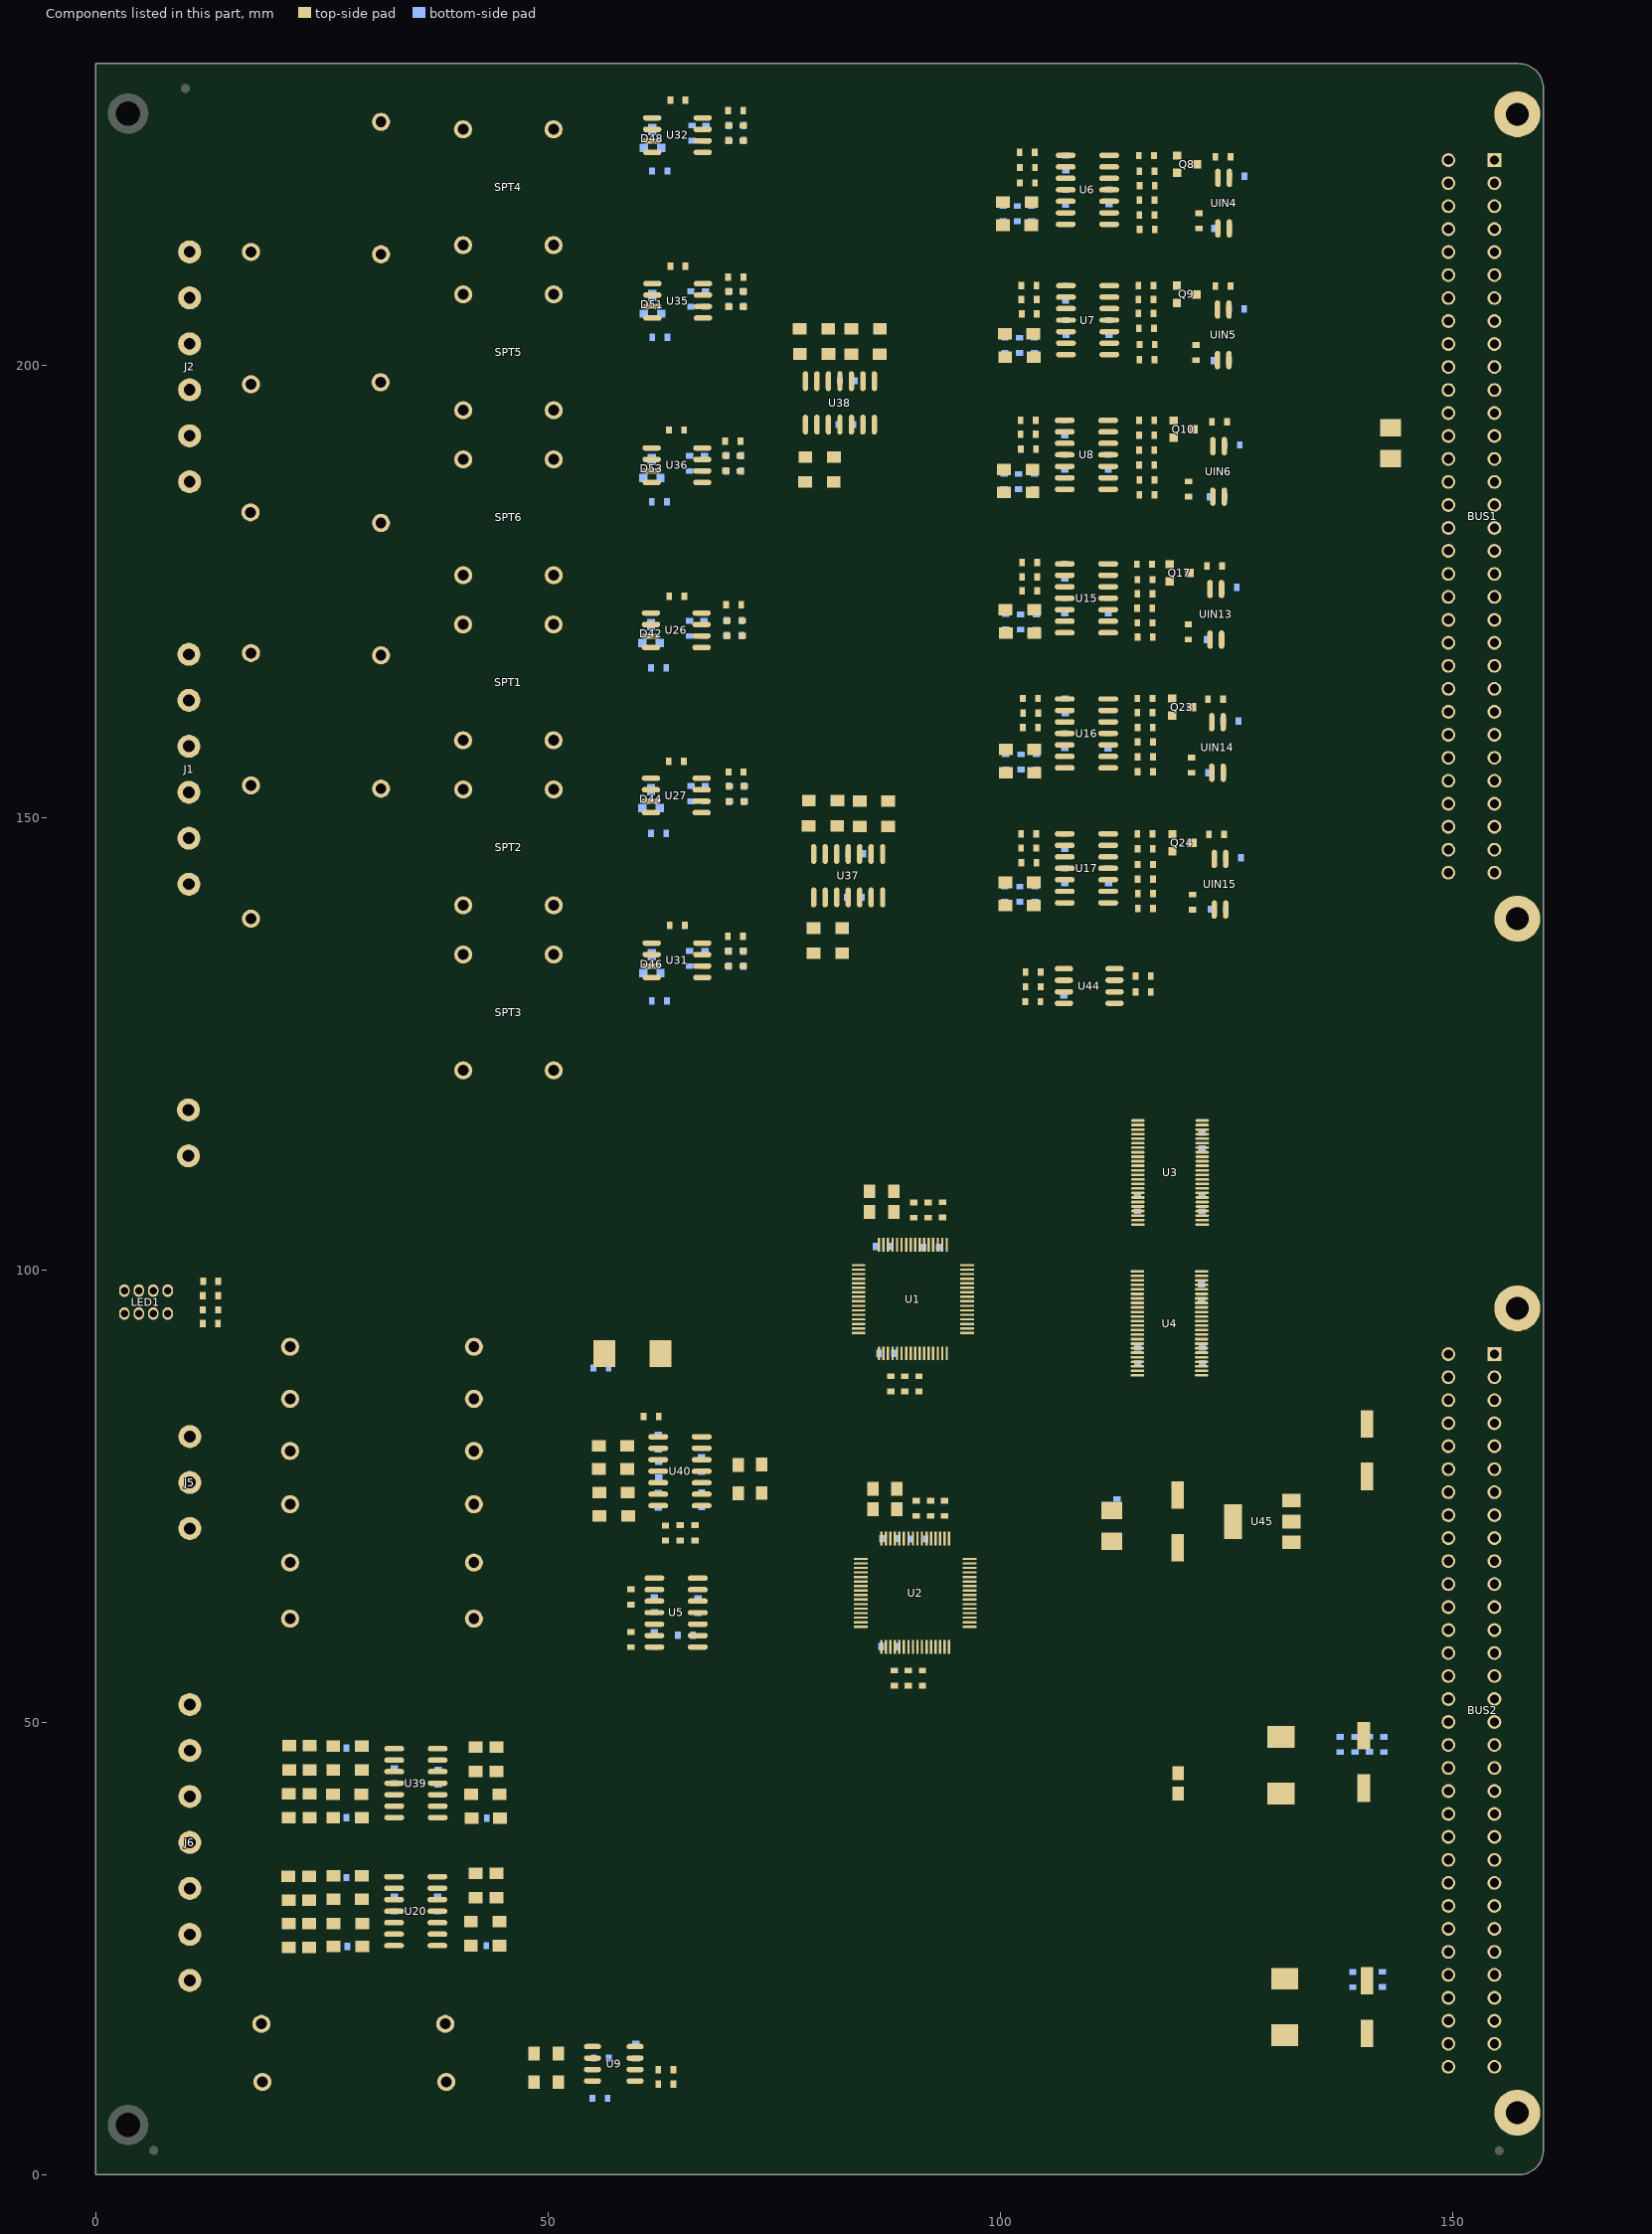
[diagram p0: the components of this part, seen from the top]
# Altium PCB MISC80584.PCBDoc (part 7 of 7)
Units mm, origin at the board's own origin, x right, y up, seen from the top; angles counter-clockwise.
Board outline 160.02 x 233.3 mm, 4 copper layers (TopLayer, GND, POWER, BottomLayer); 386 components, 266 nets, 1374 pads, 640 vias.

## Polygon pours and split planes (outlines as drawn) (continued)
AGND on TopLayer "Top Layer-No Net" (solid, remove dead copper): -1.784,125.495 -1.784,13.481 0.705,10.992 1.061,10.636 3.575,10.636 7.69,10.636 8.35,9.976 8.681,9.646 8.681,8.528 8.681,3.016 9.163,2.534 9.57,2.127 10.713,2.127 151.784,2.127 152.749,3.093 152.902,3.245 152.902,6.141 152.902,10.103 153.715,10.916 153.74,10.941 157.067,10.941 157.499,10.941 157.982,11.424 158.261,11.703 158.261,14.142 158.261,223.361 157.575,224.047 157.321,224.301 156.305,224.301 154.553,224.301 153.842,225.012 153.003,225.851 153.003,227.121 153.003,230.626 152.089,231.54 151.86,231.769 149.955,231.769 59.582,231.769 59.277,231.464 58.134,230.321 58.134,226.105 58.134,118.231 57.245,117.342 56.509,116.605 51.581,116.605 23.717,116.605 22.574,117.748 22.447,117.875 22.447,120.491 22.447,126.079 20.72,127.807 20.238,128.289 17.698,128.289 1.213,128.289 -0.514,126.562 -1.581,125.495 -1.784,125.495
GND on TopLayer "Top Layer-No Net" (solid, remove dead copper): 107.848,75.413 107.848,45.06 108.534,44.374 109.322,43.586 120.929,43.586 121.183,43.84 121.336,43.993 121.336,45.212 121.336,58.979 123.901,61.544 124.003,61.646 129.057,61.646 135.89,61.646 137.033,62.789 137.871,63.627 137.871,65.964 137.871,69.113 137.871,69.774 137.109,70.536 136.957,70.688 132.817,70.688 130.734,70.688 129.769,69.723 128.499,68.453 124.968,68.453 123.8,68.453 121.742,70.51 121.158,71.095 113.767,71.095 110.642,71.095 110.439,71.298 109.957,71.78 109.957,72.517 109.957,78.207 110.871,79.121 111.379,79.629 111.608,79.858 130.505,79.858 130.988,80.34 131.801,81.153 139.624,81.153 142.088,81.153 142.773,81.839 143.154,82.22 149.25,82.22 155.499,82.22 155.778,82.499 155.931,82.652 155.931,83.541 155.931,91.567 155.702,91.796 155.651,91.846 154.559,91.846 130.531,91.846 127.076,88.392 125.679,86.995 120.345,86.995 112.878,86.995 110.134,84.252 107.848,81.966 107.848,75.413
+15V on TopLayer "Top Layer-No Net" (solid, remove dead copper): 51.867,91.897 51.867,89.484 51.867,88.976 52.273,88.57 52.756,88.087 54.127,88.087 57.353,88.087 57.582,88.316 57.81,88.544 57.81,89.332 57.81,92.837 57.252,93.396 57.175,93.472 55.982,93.472 52.705,93.472 52.146,92.913 51.867,92.634 51.867,91.897
+5V on TopLayer "TopLayer-No Net" (solid, remove dead copper, pour order 1002): 141.072,189.56 141.072,186.665 144.018,183.718 144.094,183.642 154.432,183.642 155.346,183.642 155.6,183.896 155.956,184.252 155.956,185.293 155.956,194.869 155.55,195.275 155.346,195.478 155.296,195.529 148.615,195.529 147.447,195.529 147.168,195.25 146.888,194.97 146.888,194.513 146.888,191.338 146.685,191.135 146.304,190.754 144.856,190.754 141.453,190.754 141.224,190.525 141.072,190.373 141.072,189.56
+5V on TopLayer "TopLayer-No Net" (solid, remove dead copper, pour order 1001): 130.962,76.505 130.962,73.99 130.962,73.889 131.14,73.711 131.801,73.711 133.426,73.711 138.074,73.711 138.227,73.558 139.751,72.034 153.873,72.034 155.321,72.034 155.55,72.263 155.905,72.619 155.905,73.177 155.905,80.772 155.55,81.128 155.296,81.382 155.245,81.432 155.219,81.407 146.406,81.407 145.415,81.407 143.967,79.959 142.977,78.969 140.538,78.969 132.283,78.969 132.207,78.969 132.08,78.969 131.343,78.232 131.039,77.927 130.962,77.851 130.962,76.505
+3.3V on TopLayer "TopLayer-No Net" (solid, remove dead copper, pour order 1000): 110.642,76.429 110.642,74.143 110.642,73.482 110.642,72.923 110.642,72.72 111.049,72.314 114.046,72.314 115.138,73.406 119.888,73.406 122.301,73.406 122.987,72.72 123.419,72.288 123.419,71.73 123.419,70.587 123.825,70.18 124.308,69.698 124.689,69.698 128.295,69.698 129.337,70.739 129.972,71.374 131.877,71.374 133.172,71.374 133.299,71.501 133.375,71.577 133.375,71.704 133.375,72.923 133.274,73.025 133.223,73.076 133.172,73.127 129.997,73.127 124.257,78.867 112.192,78.867 111.506,78.867 110.769,78.13 110.668,78.029 110.642,78.003 110.642,76.454
+5VREF on TopLayer "Top Layer-No Net" (solid, remove dead copper, pour order 1000): 116.256,132.867 116.256,132.131 116.256,132.029 116.485,131.902 116.669,131.801 117.495,131.801 120.202,131.801 120.431,131.928 120.523,131.978 120.523,132.563 120.523,132.969 120.248,133.121 120.202,133.147 119.238,133.147 116.531,133.147 116.348,133.045 116.256,132.994 116.256,132.867
+15V on TopLayer "TopLayer-No Net" (solid, remove dead copper, pour order 1000): 128.397,50.47 128.397,48.26 128.397,47.549 128.397,47.447 129.032,46.812 129.057,46.787 129.235,46.609 155.372,46.609 155.524,46.609 155.575,46.609 156.337,47.371 156.54,47.574 156.54,49.428 156.54,57.633 155.854,58.318 155.6,58.572 154.788,58.572 147.955,58.572 147.168,57.785 142.926,53.543 142.545,53.162 131.445,53.162 129.997,53.162 129.515,52.68 128.397,51.562 128.397,50.47
-15V on TopLayer "TopLayer-No Net" (solid, remove dead copper, pour order 1001): 128.473,24.282 128.473,21.514 128.473,20.803 128.829,20.447 129.438,19.837 140.208,19.837 145.644,19.837 146.685,18.796 146.863,18.618 146.888,18.593 155.448,18.593 155.55,18.593 155.829,18.872 156.718,19.761 156.718,32.233 156.718,32.512 156.718,32.588 155.931,33.376 155.88,33.426 153.086,33.426 148.336,33.426 146.964,32.055 143.129,28.219 139.37,28.219 130.734,28.219 129.159,26.645 128.473,25.959 128.473,24.282
AGND on BottomLayer "Top Layer-No Net" (solid, remove dead copper): -1.778,125.508 -1.778,13.494 0.711,11.005 1.067,10.649 3.581,10.649 7.696,10.649 8.357,9.989 8.687,9.659 8.687,8.541 8.687,3.029 9.169,2.547 9.576,2.14 10.719,2.14 151.79,2.14 152.756,3.106 152.908,3.258 152.908,6.154 152.908,10.116 153.721,10.929 153.746,10.954 157.074,10.954 157.505,10.954 157.988,11.437 158.267,11.716 158.267,14.155 158.267,223.374 157.582,224.06 157.328,224.314 156.312,224.314 154.559,224.314 153.848,225.025 153.01,225.864 153.01,227.134 153.01,230.639 152.095,231.553 151.867,231.782 149.962,231.782 59.588,231.782 59.284,231.477 58.141,230.334 58.141,226.118 58.141,118.244 57.252,117.355 56.515,116.618 51.587,116.618 23.724,116.618 22.581,117.761 22.454,117.888 22.454,120.504 22.454,126.092 20.726,127.82 20.244,128.302 17.704,128.302 1.219,128.302 -0.508,126.575 -1.575,125.508 -1.778,125.508
+5VREF on BottomLayer "Top Layer-No Net" (solid, remove dead copper, pour order 1001): 118.694,132.994 118.694,132.156 118.77,132.08 119.05,131.801 119.532,131.801 120.548,131.801 120.752,132.004 120.828,132.08 120.828,132.436 120.828,133.426 120.625,133.629 120.498,133.756 120.193,133.756 119.964,133.756 119.761,133.553 119.558,133.35 119.38,133.35 118.897,133.35 118.77,133.223 118.694,133.147 118.694,133.02
+15V on BottomLayer "TopLayer-No Net" (solid, remove dead copper, pour order 1002): 136.754,49.911 136.754,48.336 136.906,48.184 137.058,48.031 137.084,48.057 141.351,48.057 142.824,48.057 142.9,48.133 143.002,48.235 143.002,48.463 143.002,51.206 142.418,51.791 142.265,51.943 140.843,51.943 138.201,51.943 138.024,51.765 136.754,50.495 136.754,49.911
-15V on BottomLayer "TopLayer-No Net" (solid, remove dead copper, pour order 1003): 138.227,24.536 138.227,22.327 138.324,22.2 138.558,21.895 139.025,21.895 142.819,21.895 143.014,22.149 143.053,22.2 143.053,22.555 143.053,24.689 142.644,25.222 138.752,25.222 138.227,24.536
AGND on GND (split plane): 157.495,232.808 157.686,232.782 157.874,232.741 158.058,232.683 158.236,232.609 158.407,232.52 158.569,232.416 158.722,232.299 158.864,232.169 158.995,232.027 159.112,231.874 159.216,231.711 159.305,231.54 159.378,231.362 159.436,231.178 159.478,230.99 159.503,230.799 159.511,230.621 159.51,230.607 159.51,221.643 125.578,221.643 125.511,221.634 125.45,221.608 125.396,221.568 120.469,216.64 120.428,216.587 120.403,216.525 120.394,216.459 120.394,126.116 114.092,119.814 95.072,119.814 95.006,119.805 94.962,119.787 94.944,119.78 94.891,119.739 89.354,114.202 89.313,114.149 89.288,114.087 89.279,114.021 89.279,102.798 88.82,102.34 88.78,102.287 88.754,102.225 88.745,102.159 88.745,101.224 88.26,100.739 87.152,100.739 86.567,101.324 86.513,101.365 86.452,101.39 86.385,101.399 84.785,101.399 84.719,101.39 84.657,101.365 84.604,101.324 84.563,101.271 84.554,101.249 83.791,100.486 83.751,100.433 83.725,100.371 83.716,100.305 83.716,87.046 83.725,86.979 83.751,86.918 83.791,86.865 89.66,80.996 89.66,68.762 89.378,68.481 84.125,68.481 84.058,68.472 83.997,68.446 83.944,68.406 80.388,64.85 80.347,64.796 80.321,64.735 80.313,64.668 80.313,55.829 80.321,55.763 80.347,55.701 80.388,55.648 80.402,55.637 80.413,55.623 90.725,45.31 90.779,45.27 90.84,45.244 90.907,45.235 118.364,45.235 118.43,45.244 118.492,45.27 118.545,45.31 139.273,66.038 159.51,66.038 159.51,2.743 159.511,2.729 159.503,2.551 159.478,2.36 159.436,2.171 159.378,1.988 159.305,1.809 159.216,1.639 159.112,1.476 158.995,1.323 158.864,1.181 158.722,1.051 158.569,0.933 158.407,0.83 158.236,0.741 158.058,0.667 157.874,0.609 157.686,0.567 157.495,0.542 157.316,0.534 157.302,0.536 0.51,0.536 0.51,129.669 0.864,130.023 23.825,130.023 24.46,129.388 24.46,119.659 25.603,118.516 44.577,118.516 44.679,118.618 44.679,232.029 45.464,232.814 157.302,232.814 157.316,232.815
GND on GND (split plane): 159.51,66.55 139.167,66.55 139.1,66.541 139.039,66.516 138.985,66.475 118.258,45.748 91.013,45.748 80.825,55.935 80.825,64.562 84.231,67.968 89.484,67.968 89.551,67.977 89.612,68.003 89.665,68.043 90.097,68.475 90.138,68.528 90.163,68.59 90.172,68.656 90.172,81.102 90.163,81.169 90.145,81.212 90.138,81.23 90.097,81.283 84.229,87.152 84.229,100.198 84.917,100.887 86.279,100.887 86.865,100.301 86.918,100.261 86.936,100.253 86.979,100.235 87.046,100.226 88.367,100.226 88.433,100.235 88.495,100.261 88.548,100.301 89.183,100.936 89.223,100.989 89.242,101.033 89.249,101.051 89.258,101.117 89.258,102.053 89.716,102.511 89.757,102.564 89.77,102.595 89.782,102.626 89.791,102.692 89.791,113.914 95.178,119.302 114.198,119.302 114.265,119.31 114.326,119.336 114.38,119.377 120.831,125.828 120.872,125.881 120.897,125.943 120.906,126.009 120.906,216.353 125.684,221.13 159.51,221.13
+15V on POWER (split plane): 313 vertices, not listed, extent 27.917,11.483 159.511,232.815
-15V on POWER (split plane): 188 vertices, not listed, extent 0.51,0.534 159.511,232.814
+5V on POWER (split plane): 189 vertices, not listed, extent 77.955,39.499 159.51,215.898
+3.3V on POWER (split plane): 120.673,105.105 120.682,105.039 120.708,104.977 120.748,104.924 124.636,101.037 124.636,99.014 123.719,98.097 121.336,98.097 121.269,98.088 121.226,98.07 121.208,98.063 121.155,98.022 120.113,96.981 120.073,96.927 120.047,96.866 120.038,96.799 120.038,76.581 120.04,76.568 120.038,76.556 120.038,71.15 100.783,51.894 89.26,51.894 87.785,53.37 87.785,56.587 93.425,62.227 93.465,62.28 93.491,62.341 93.5,62.408 93.5,72.746 93.491,72.812 93.473,72.856 93.465,72.874 93.425,72.927 91.315,75.036 91.315,76.657 91.306,76.724 91.281,76.785 91.24,76.838 88.14,79.938 88.14,89.2 89.894,90.954 89.935,91.007 89.942,91.025 89.96,91.069 89.969,91.135 89.969,97.328 93.577,100.936 93.618,100.989 93.625,101.007 93.643,101.051 93.652,101.117 93.652,104.394 93.643,104.46 93.625,104.504 93.618,104.522 93.577,104.575 92.536,105.617 92.482,105.657 92.421,105.683 92.354,105.692 83.263,105.692 83.263,108.301 92.105,117.143 120.673,117.143

## Keep-outs
KeepOutLayer:
  lines w0.127: 4.394,130.073 cw(c4.394,130.835) 4.394,131.597 24.663,131.597 26.086,130.175 26.086,120.345 26.391,120.04 35.687,120.04 43.155,120.04 43.155,126.086 cw(c43.917,126.086) 44.679,126.086 44.679,118.516 35.687,118.516 25.578,118.516 24.46,119.634 24.46,129.362 23.749,130.073 4.42,130.073 ; 37.109,228.016 43.155,228.016 43.155,220.548 ccw(c43.917,220.548) 44.679,220.548 44.679,229.54 37.109,229.54 ; 37.16,228.016 cw(c37.16,228.778) 37.16,229.54 ; 43.155,131.928 ccw(c43.917,131.928) 44.679,131.928 44.679,143.815 ccw(c43.917,143.815) 43.155,143.815 43.155,131.928 ; 43.155,149.835 ccw(c43.917,149.835) 44.679,149.835 44.679,161.722 ccw(c43.917,161.722) 43.155,161.722 43.155,149.835 ; 43.155,165.837 ccw(c43.917,165.837) 44.679,165.837 44.679,180.797 ccw(c43.917,180.797) 43.155,180.797 43.155,173.228 43.155,165.837 ; 43.155,186.639 ccw(c43.917,186.639) 44.679,186.639 44.679,198.526 ccw(c43.917,198.526) 43.155,198.526 43.155,186.639 ; 43.155,204.546 ccw(c43.917,204.546) 44.679,204.546 44.679,216.433 ccw(c43.917,216.433) 43.155,216.433 43.155,204.546
  lines w0.254: 0,0.025 157.302,0.025 ccw(c157.302,2.743) 160.02,2.743 160.02,230.607 ccw(c157.302,230.607) 157.302,233.324 0,233.324 0,0.025

## Other copper
GND (plane layer: these items are gaps in the copper):
  region: 0.127,231.902 0.051,231.826 0.051,129.21 0.864,130.023 23.825,130.023 24.46,129.388 24.46,119.659 25.603,118.516 44.577,118.516 44.679,118.618 44.679,232.029 46.05,233.401 45.745,233.705 0.965,233.705 0.127,232.867
  lines w0.508: 80.569,55.829 80.569,64.668 84.125,68.224 89.484,68.224 89.916,68.656 89.916,81.102 83.972,87.046 83.972,100.305 84.785,101.117 ; 80.594,55.804 90.907,45.491 118.364,45.491 139.167,66.294 159.868,66.294 ; 84.785,101.143 86.385,101.143 87.046,100.482 88.367,100.482 89.002,101.117 89.002,102.159 89.535,102.692 89.535,114.021 95.072,119.558 114.198,119.558 120.65,126.009 120.65,216.459 125.578,221.386 159.842,221.386
POWER (plane layer: these items are gaps in the copper):
  region: 0.127,231.902 0.051,231.826 0.051,129.21 0.864,130.023 23.825,130.023 24.46,129.388 24.46,119.659 25.603,118.516 44.577,118.516 44.679,118.618 44.679,232.029 46.05,233.401 45.745,233.705 0.965,233.705 0.127,232.867
  lines w0.508: 65.253,148.565 71.399,142.418 83.541,142.418 85.141,140.818 85.141,137.82 83.21,135.89 73,135.89 71.679,137.211 66.523,137.211 64.287,134.976 64.287,110.719 64.287,94.844 69.367,89.764 69.367,62.255 68.529,61.417 66.015,61.417 62.255,65.176 62.255,86.182 54.508,93.929 43.942,93.929 27.661,77.648 27.661,29.896 29.947,27.61 34.874,27.61 37.668,30.404 37.668,44.094 38.557,44.983 42.748,44.983 45.974,41.758 45.974,17.348 52.095,11.227 122.352,11.227 145.542,34.417 159.791,34.417 ; 65.278,148.565 62.636,151.206 62.636,220.98 67.818,226.162 69.926,226.162 74.371,221.717 74.371,215.214 81.763,207.823 ; 81.788,207.797 83.82,205.765 83.82,199.212 78.613,194.005 78.613,190.805 80.721,188.697 87.452,188.697 89.992,191.237 89.992,218.034 92.786,220.828 108.687,220.828 109.652,219.862 ; 83.007,105.512 83.007,108.407 91.999,117.399 120.904,117.399 ; 109.652,219.761 109.652,144.678 111.608,142.723 ; 111.582,142.723 115.443,142.723 115.926,143.205 ; 115.849,143.129 116.713,143.993 116.713,220.523 ; 116.637,233.426 116.688,233.375 116.688,220.574 ; 120.294,76.556 120.294,71.044 100.889,51.638 89.154,51.638 87.528,53.264 87.528,56.693 93.243,62.408 93.243,72.746 91.059,74.93 91.059,76.657 87.884,79.832 87.884,89.306 89.713,91.135 89.713,97.434 93.396,101.117 93.396,104.394 92.354,105.435 83.083,105.435 77.699,100.051 77.699,44.044 82.499,39.243 112.573,39.243 139.649,66.319 160.071,66.319 ; 120.294,76.581 120.294,96.799 121.336,97.841 123.825,97.841 124.892,98.908 124.892,101.143 120.929,105.105 120.929,117.424 123.266,119.761 ; 123.165,119.659 123.266,119.761 ; 159.893,216.154 125.197,216.154 ; 160.299,216.154 125.197,216.154 ; 123.266,119.761 123.266,139.624 124.409,140.767 127.737,140.767 128.829,141.859 128.829,148.336 127.737,149.428 124.485,149.428 123.266,150.647 123.266,155.169 123.85,155.753 126.873,155.753 128.321,157.201 128.321,163.297 127.356,164.262 124.308,164.262 123.266,165.303 123.266,170.358 123.876,170.967 127.737,170.967 128.88,172.11 128.88,177.902 127.508,179.273 123.876,179.273 123.266,179.883 123.266,185.522 123.825,186.08 126.822,186.08 128.346,187.604 128.346,193.319 127.178,194.488 124.13,194.488 123.266,195.351 123.266,200.584 124.206,201.524 127.787,201.524 128.778,202.514 128.778,209.067 127.203,210.642 124.308,210.642 123.266,211.684 123.266,214.224 ; 123.266,214.224 125.197,216.154 ; 123.266,214.224 125.197,216.154

## Silkscreen, mask and mechanical layers (free items; w line width, h text height)
Mechanical1:
  lines w0.254: 0.051,225.323 7.01,225.323 7.01,233.324 ; 0.062,8.023 7.021,8.023 7.021,0.049